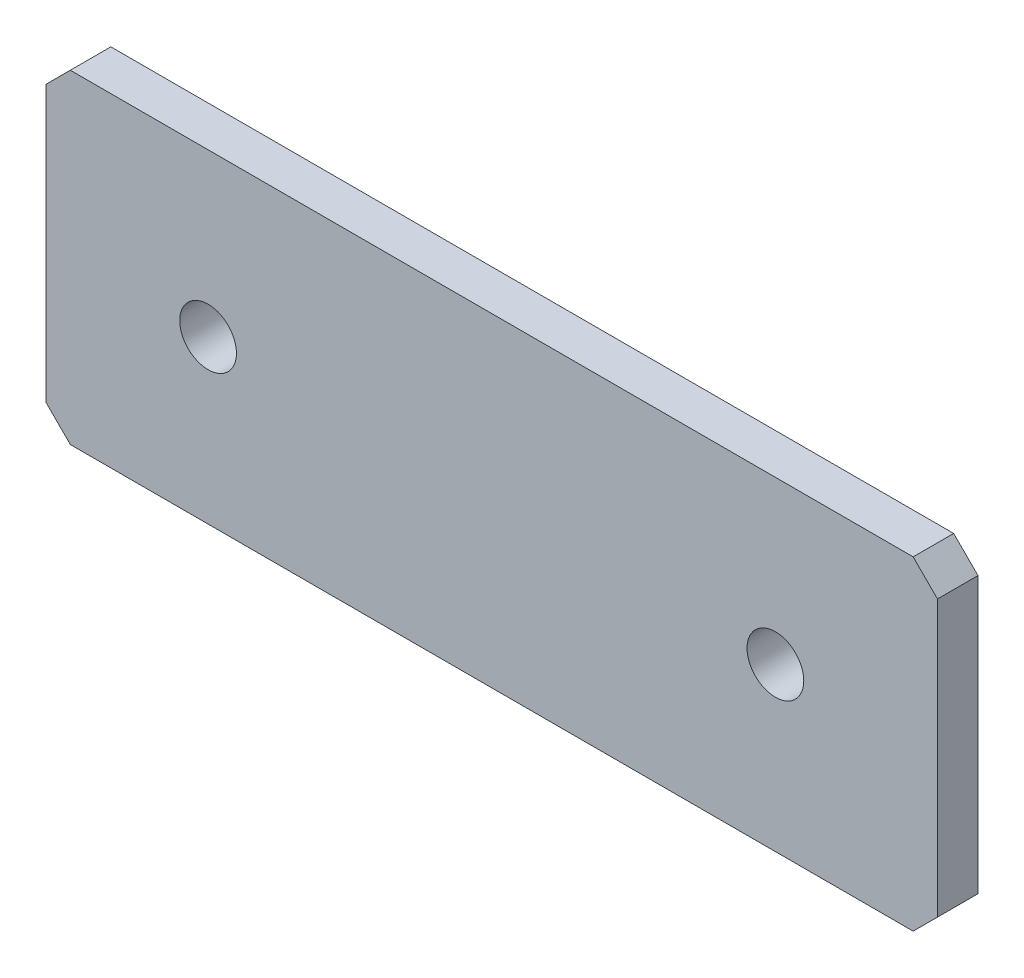
SolidWorks part; units mm, degrees
material "1023 碳钢板 (SS)"
ref_plane "Front Plane" through (0, 0, 0) normal (0, 0, 1) x (1, 0, 0)
ref_plane "Top Plane" through (0, 0, 0) normal (0, 1, 0) x (1, 0, 0)
ref_plane "Right Plane" through (0, 0, 0) normal (1, 0, 0) x (0, 0, -1)
sketch "Sketch1" plane through (0, 0, 0) normal (0, 0, 1) x (1, 0, 0)
  line L1 (55, 20) -> (-55, 20)
  line L2 (55, 20) -> (55, -20)
  line L3 (55, -20) -> (-55, -20)
  line L4 (-55, 20) -> (-55, -20)
  line L5 (55, 20) -> (-55, -20) construction
  line L6 (55, -20) -> (-55, 20) construction
  circle A0 centre (-35, 0) radius 3.5
  circle A1 centre (35, 0) radius 3.5
  point P0 (0, 0)
  dimension "D3" = 7
  dimension "D4" = 20
  dimension "D5" = 70
  dimension "D1" = 110
  dimension "D2" = 40
extrude "Boss-Extrude1" add sketch "Sketch1" along normal blind 5 contours A0 | A1 | L2 L1 L4 L3
chamfer "Chamfer1" distance 3 angle 45 4 edges at (-55, 20, 2.5) (-55, -20, 2.5) (55, -20, 2.5) (55, 20, 2.5)
